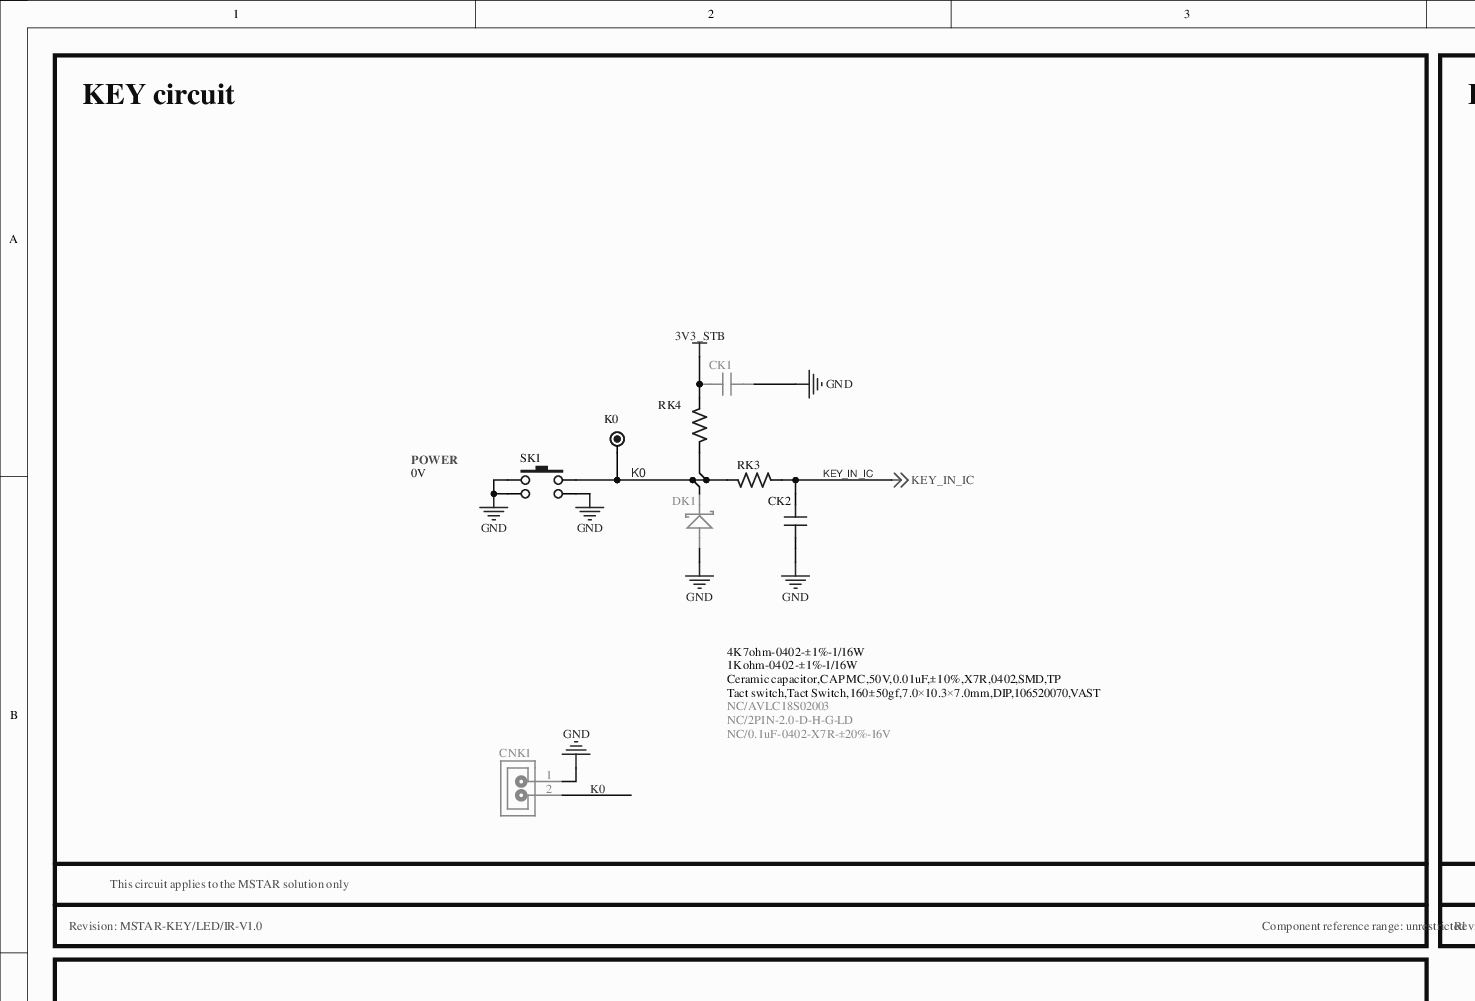
[diagram p0: MISC116569-8.SchDoc, top left]
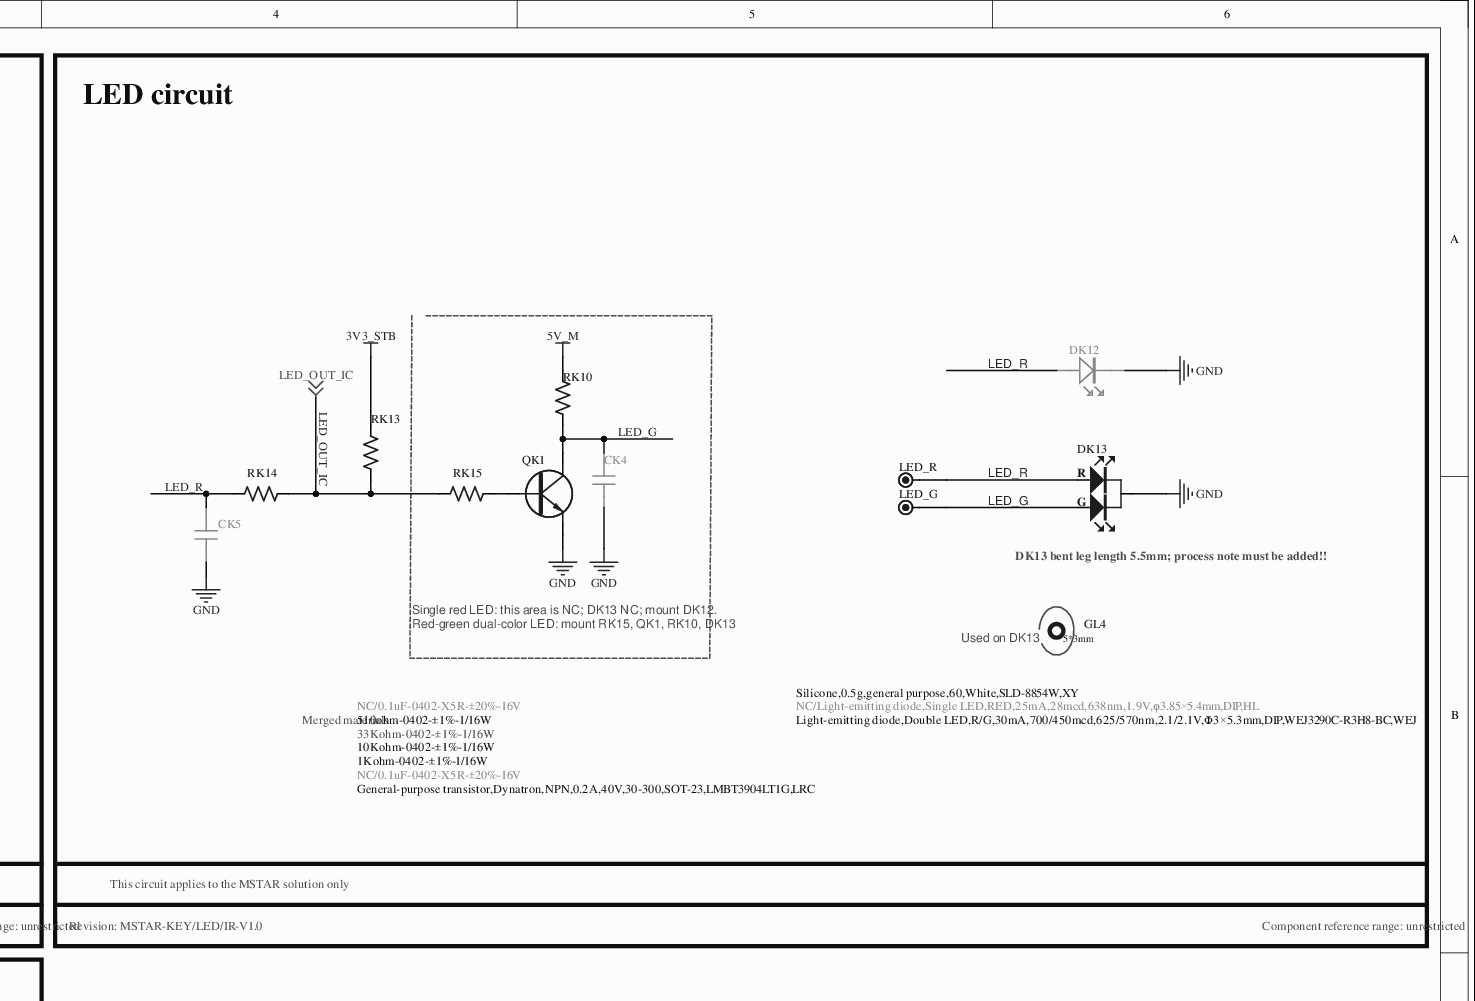
[diagram p1: MISC116569-8.SchDoc, top right]
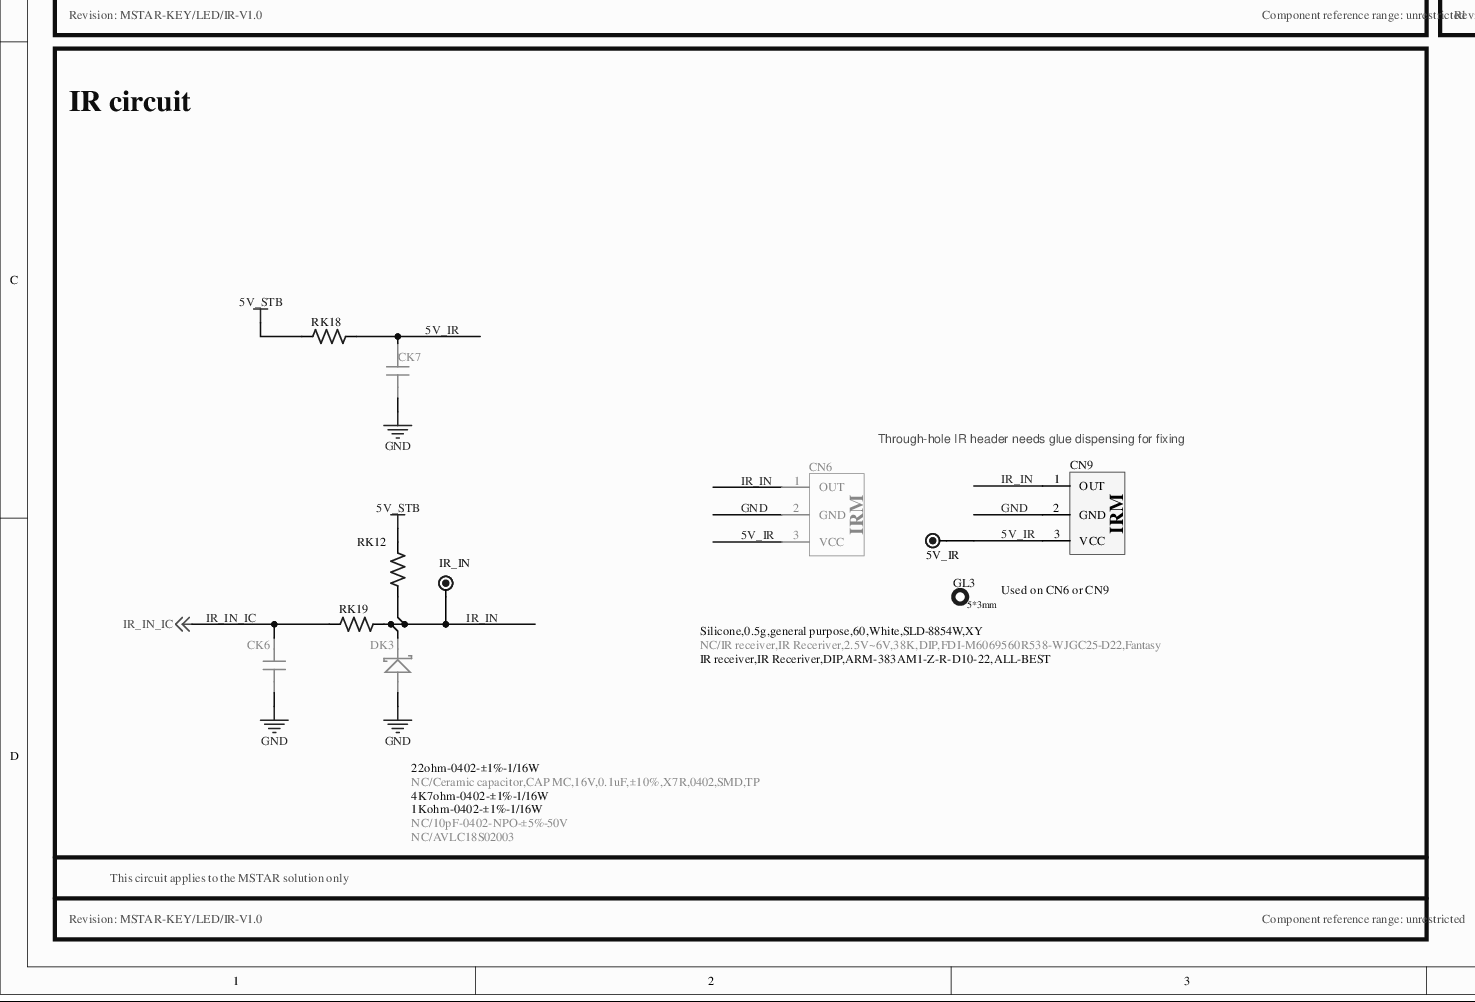
[diagram p2: MISC116569-8.SchDoc, bottom left]
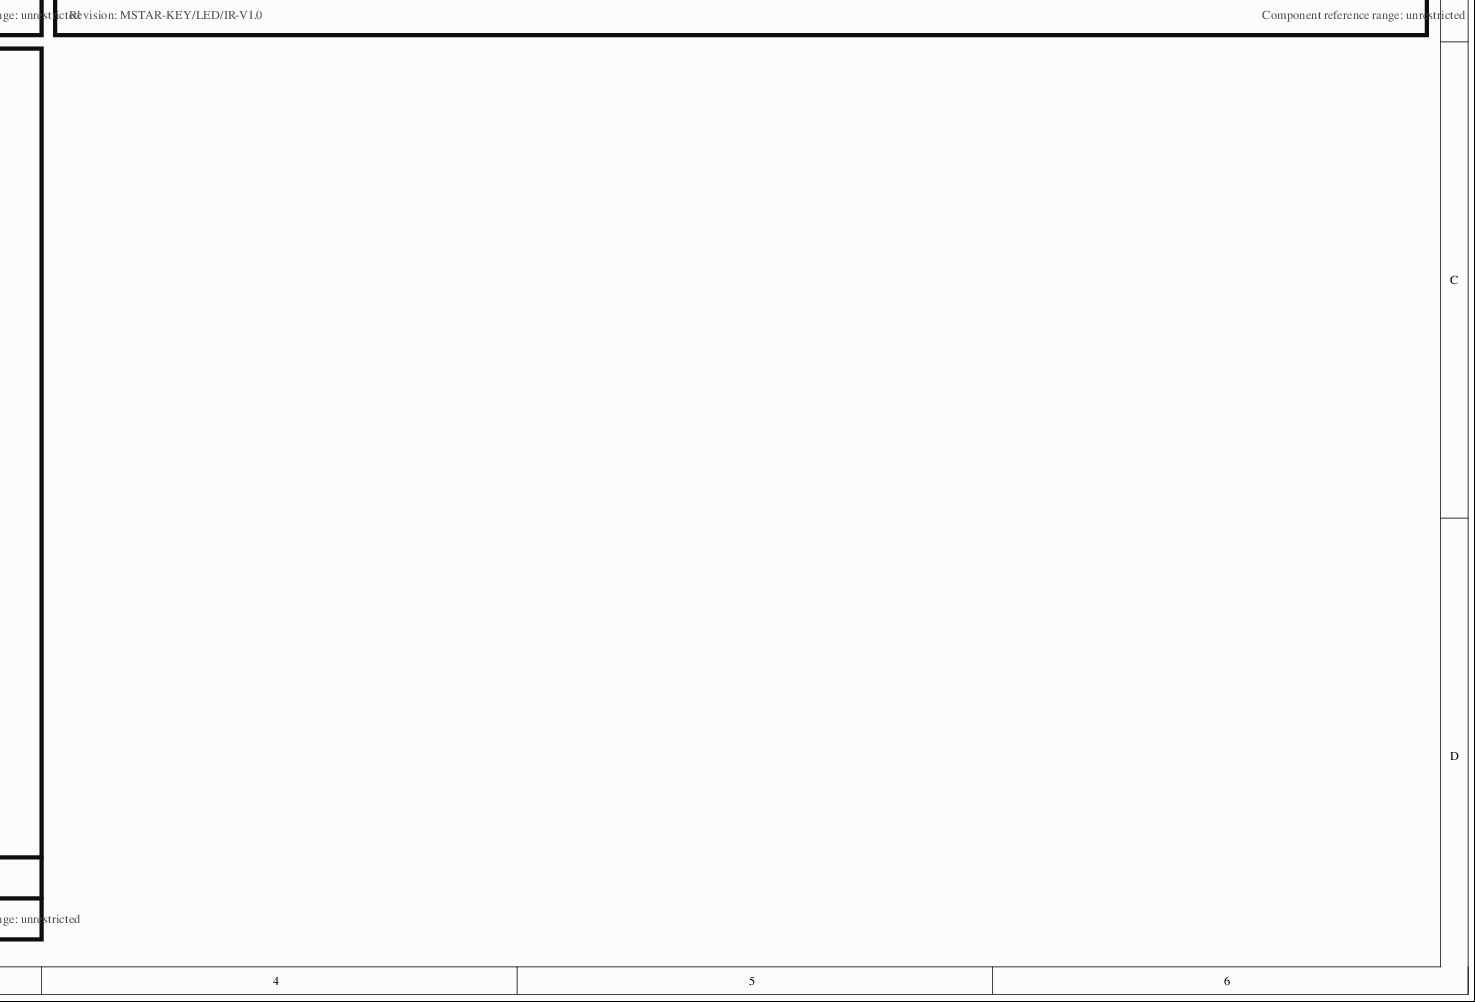
[diagram p3: MISC116569-8.SchDoc, bottom right]
# Altium project MISC116569-15.PrjPCB (part 4 of 8)

## Sheet MISC116569-8.SchDoc
size 528 x 353 mm

### Parts
5V_IR  TEST  SL  [TP]  (value not drawn)
CK1  NC/0.1uF-0402-X7R-±20%-16V  [C0402]
CK2  Ceramic capacitor,CAP MC,50V,0.01uF,±10%,X7R,0402,SMD,TP  [C0402]
CK4  NC/0.1uF-0402-X5R-±20%-16V  [C0402]
CK5  NC/0.1uF-0402-X5R-±20%-16V  [C0402]
CK6  NC/10pF-0402-NPO-±5%-50V  [C0402]
CK7  NC/Ceramic capacitor,CAP MC,16V,0.1uF,±10%,X7R,0402,SMD,TP  [C0402]
CN6  NC/IR receiver,IR Receriver,2.5V~6V,38K,DIP,FDI-M6069560R538-WJGC25-D22,Fantasy  [REMOTE-VD-9]
CN9  IR receiver,IR Receriver,DIP,ARM-383AM1-Z-R-D10-22,ALL-BEST  [REMOTE-VD-6]
CNK1  NC/2PIN-2.0-D-H-G-LD  [SIP2/2.0D-1]
DK1  NC/AVLC18S02003  [DIODE-S0402]
DK3  NC/AVLC18S02003  [DIODE-S0402]
DK12  NC/Light-emitting diode,Single LED,RED,25mA,28mcd,638nm,1.9V,φ3.85×5.4mm,DIP,HL  [LED-HD-6]
DK13  Light-emitting diode,Double LED,R/G,30mA,700/450mcd,625/570nm,2.1/2.1V,Φ3×5.3mm,DIP,WEJ3290C-R3H8-BC,WEJ  [LED-HD-5]
GL3  Silicone,0.5g,general purpose,60,White,SLD-8854W,XY  [Silica gel-5*3]
GL4  Silicone,0.5g,general purpose,60,White,SLD-8854W,XY  [Silica gel-5*3]
IR_IN  TEST  SL  [TP]  (value not drawn)
K0  TEST  SL  [TP]  (value not drawn)
LED_G  TEST  SL  [TP]  (value not drawn)
LED_R  TEST  SL  [TP]  (value not drawn)
QK1  General-purpose transistor,Dynatron,NPN,0.2A,40V,30-300,SOT-23,LMBT3904LT1G,LRC  [SOT-23]
RK3  1Kohm-0402-±1%-1/16W  [R0402]
RK4  4K7ohm-0402-±1%-1/16W  [R0402]
RK10  1Kohm-0402-±1%-1/16W  [R0402]
RK12  4K7ohm-0402-±1%-1/16W  [R0402]
RK13  33Kohm-0402-±1%-1/16W  [R0402]
RK14  510ohm-0402-±1%-1/16W  [R0402]
RK15  10Kohm-0402-±1%-1/16W  [R0402]
RK18  22ohm-0402-±1%-1/16W  [R0402]
RK19  1Kohm-0402-±1%-1/16W  [R0402]
SK1  Tact switch,Tact Switch,160±50gf,7.0×10.3×7.0mm,DIP,106520070,VAST  [KEY-HD-6]

### Blocks framed on the sheet
KEY circuit: CK1 CK2 CNK1 DK1 K0 RK3 RK4 SK1
LED circuit: CK4 CK5 DK12 DK13 GL4 LED_G LED_R QK1 RK10 RK13-RK15
IR circuit: 5V_IR CK6 CK7 CN6 CN9 DK3 GL3 IR_IN RK12 RK18 RK19

### Nets
3V3_STB: CK1.2 RK4.2 RK13.2
5V_M: RK10.2
5V_STB: RK12.2 RK18.2
GND: CK1.1 CK2.2 CK4.2 CK5.2 CK6.1 CK7.2 CN6.2(GND) CN9.2(GND) CNK1.1 DK1.A DK3.A DK12.K DK13.2 QK1.E SK1.1 SK1.3 SK1.4
5V_IR: 5V_IR.1 CK7.1 CN6.3(VCC) CN9.3(VCC) RK18.1
IR_IN: CN6.1(OUT) CN9.1(OUT) DK3.K IR_IN.1 RK12.1 RK19.1
IR_IN_IC: CK6.2 RK19.2 ; off-sheet IR_IN_IC
K0: CNK1.2 DK1.K K0.1 RK3.2 RK4.1 SK1.2
KEY_IN_IC: CK2.1 RK3.1 ; off-sheet KEY_IN_IC
LED_G: CK4.1 DK13.1 LED_G.1 QK1.C RK10.1
LED_OUT_IC: RK13.1 RK14.1 RK15.2 ; off-sheet LED_OUT_IC
LED_R: CK5.1 DK12.A DK13.3 LED_R.1 RK14.2
NetQK1_B: QK1.B RK15.1

### Notes on the sheet
- POWER
- 0V
- (near DK13) DK13 bent leg length 5.5mm; process note must be added!!
- Single red LED: this area is NC; DK13 NC; mount DK12.
- Red-green dual-color LED: mount RK15, QK1, RK10, DK13
- (near GL4) Used on DK13
- Merged materials
- This circuit applies to the MSTAR solution only
- Revision: MSTAR-KEY/LED/IR-V1.0
- Component reference range: unrestricted
- (near CN9) Through-hole IR header needs glue dispensing for fixing
- Used on CN6 or CN9

### Library data of the parts
CK1 = 0.1uF-0402-Y5V-+80%-20%-16V-D
CK2 = 0.01uF-0402-X7R-±10%-50V-D
CK4 CK5 = 0.1uF-0402-X5R-±20%-16V-D
CK6 = 10pF-0402-NPO-±5%-50V-D
CK7 = 1uF-0402-X5R-±20%-6.3V-D
CN6 = 004.008.0000361-DHMI: IR receiver,IR Receriver,2.5V~6V,38K,DIP,FDI-M6069560R538-WJGC25-D22,Fantasy-DHMI
CN9 = 004.008.0000501-DHMI: IR receiver,IR Receriver,DIP,ARM-383AW1-Z-R-D10-22,ALL-BEST-DHMI
CNK1 = 2PIN-2.0-D-H-G-B-DHMI: Socket
DK1 DK3 = AVLC18S02003-D
DK12 = 发光二极管,Single LED,RED,25mA,28mcd,638nm,1.9V,φ3.85×5.4mm,DIP,HL-DLMI
DK13 = WEJ3290C-R3H8-BC(红、绿)-高亮-DLMI
GL3 GL4 = 005.002.0000011-D-5*3mm: Silicone,0.5g,general purpose,60,White,SLD-8854W,XY-D
QK1 = LMBT3904LT1G-D-NPN: Q-NPN-#-#-#
RK3 RK10 = 1Kohm-0402-±5%-1/16W-D
RK4 = 4K7ohm-0402-±1%-1/16W-D
RK12 = 4K7ohm-0402-±5%-1/16W-D
RK13 = 33Kohm-0402-±5%-1/16W-D
RK14 = 510ohm-0402-±5%-1/16W-D
RK15 = 10Kohm-0402-±5%-1/16W-D
RK18 RK19 = 100ohm-0402-±5%-1/16W-D
SK1 = 轻触开关,Tact Switch,160±50gf,7.0×10.3×7.0mm,DIP,KFC-A06-E-4-7.5/4(R),YK-DLMI

## Sheet MISC116569-9.SchDoc
size 215 x 228 mm
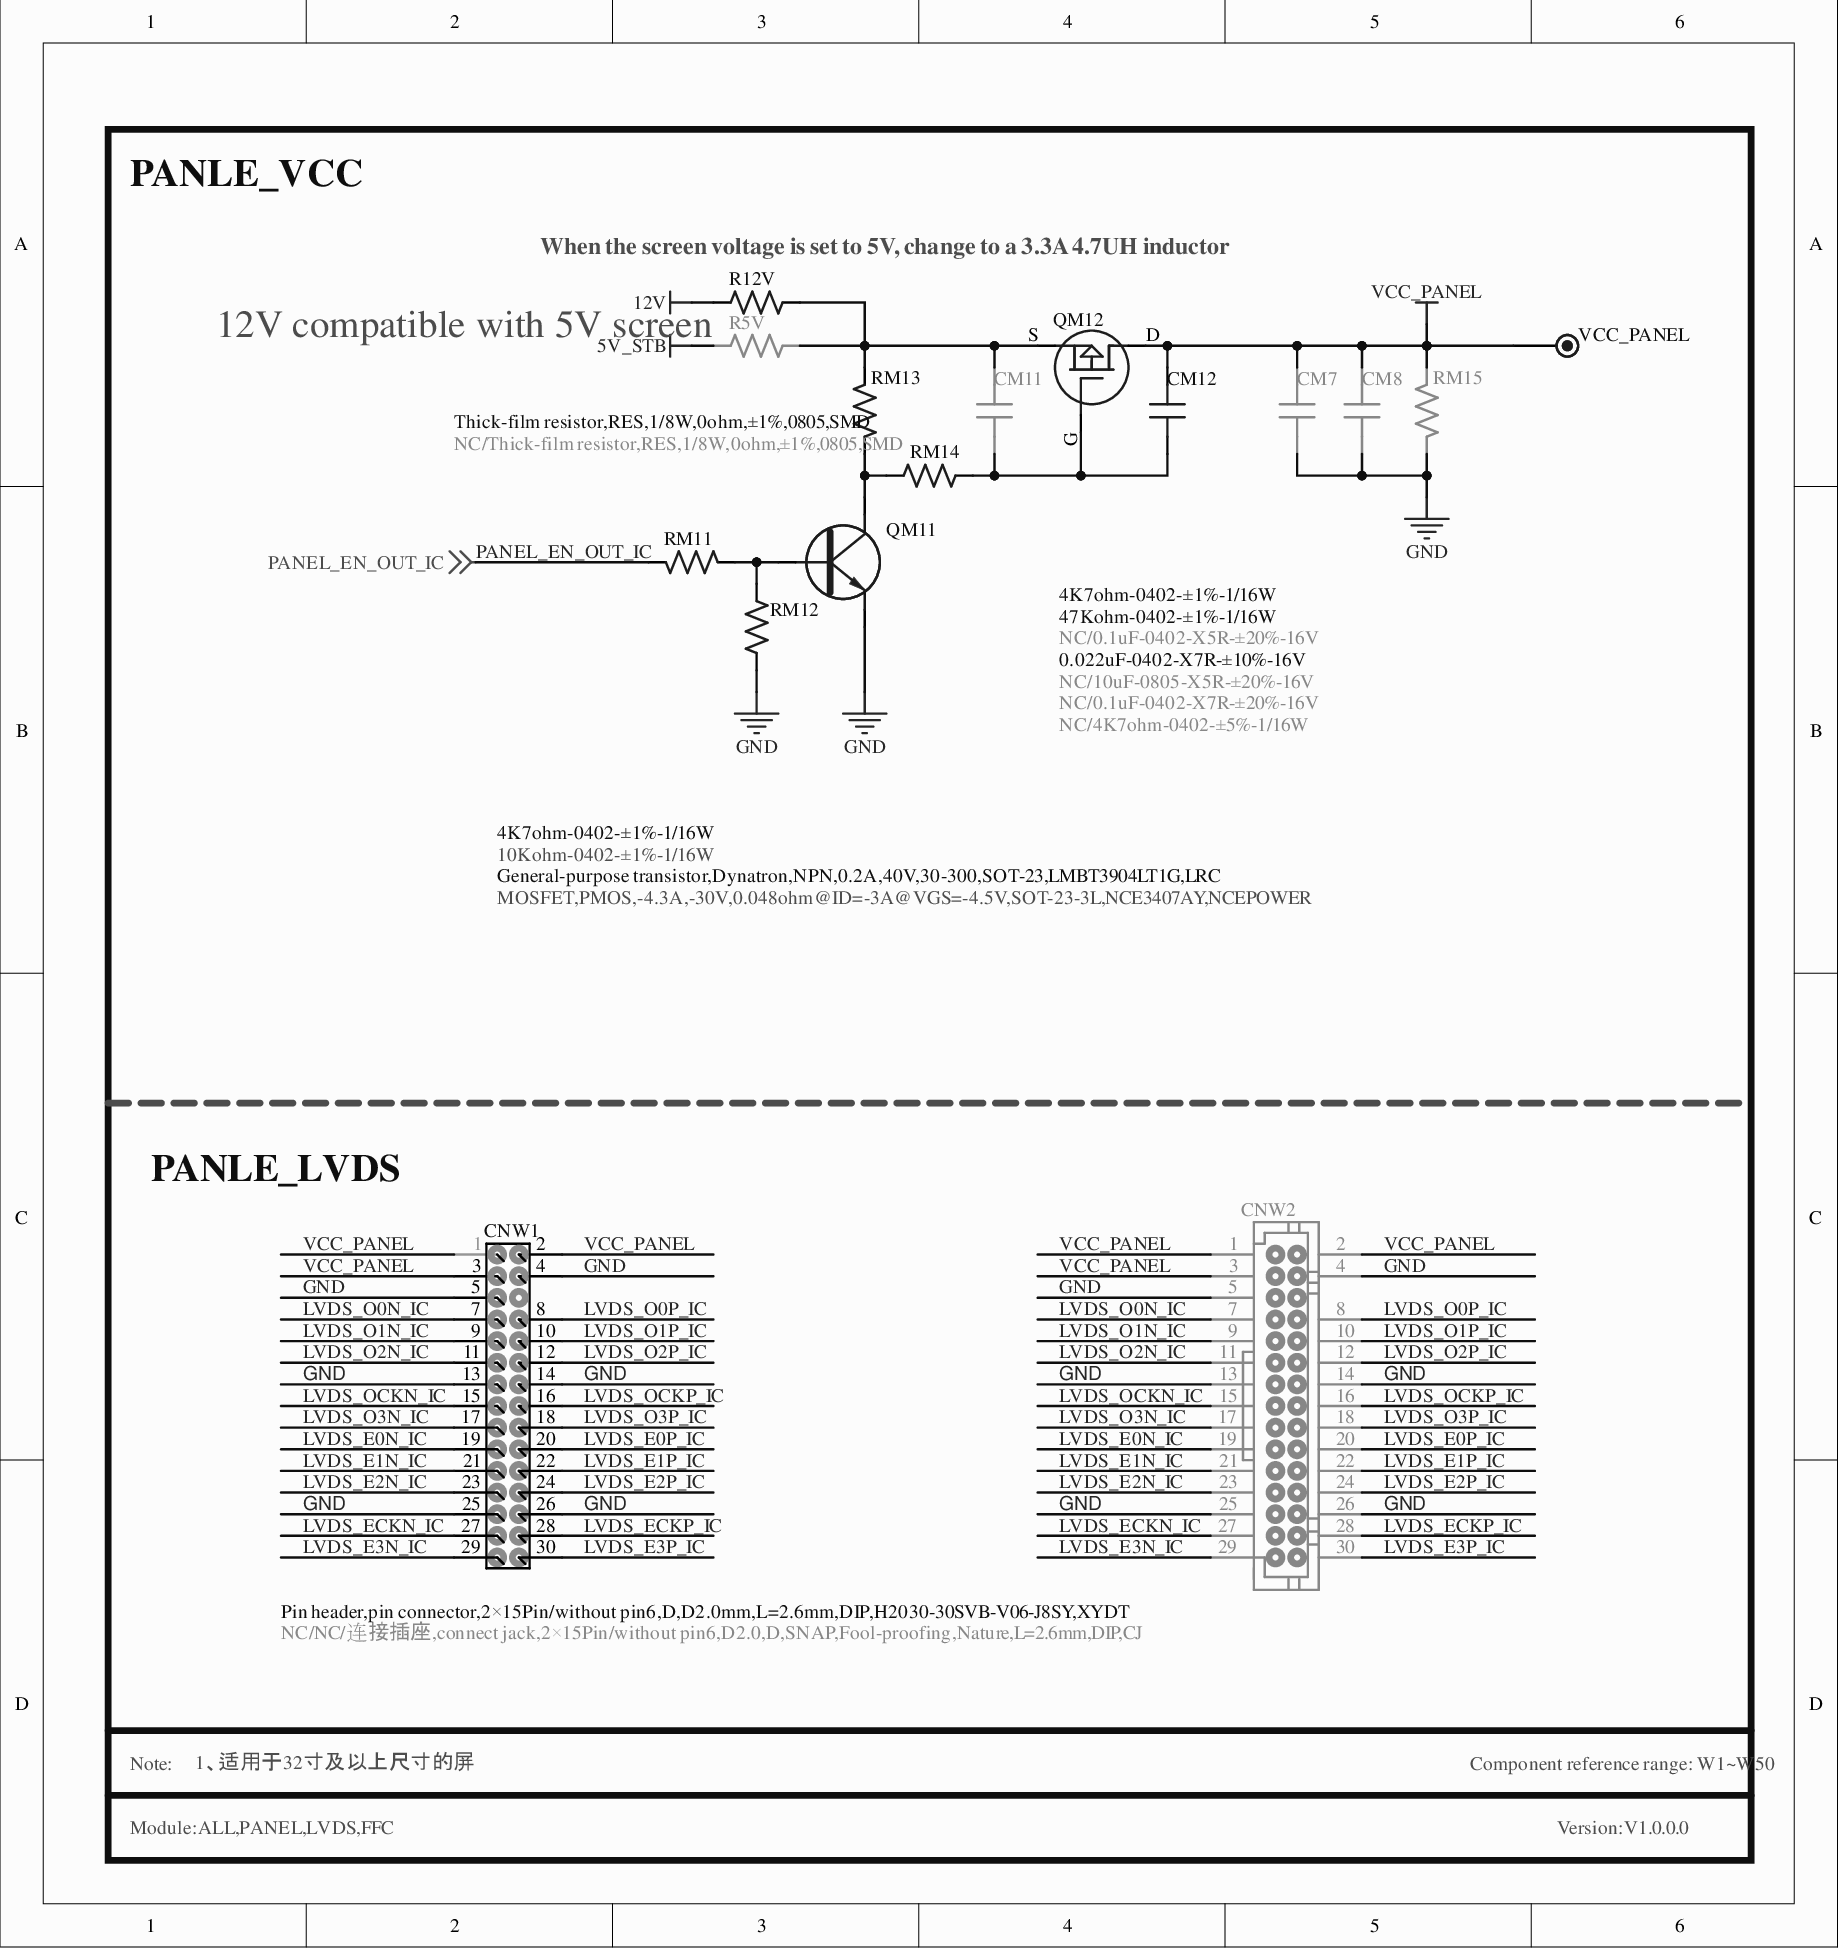
[diagram p4: MISC116569-9.SchDoc]

### Parts
CM7  NC/10uF-0805-X5R-±20%-16V  [C0805]
CM8  NC/0.1uF-0402-X7R-±20%-16V  [C0402]
CM11  NC/0.1uF-0402-X5R-±20%-16V  [C0402]
CM12  0.022uF-0402-X7R-±10%-16V  [C0402]
CNW1  Pin header,pin connector,2×15Pin/without pin6,D,D2.0mm,L=2.6mm,DIP,H2030-30SVB-V06-J8SY,XYDT  [SIP2*15/2.0D-2]
CNW2  NC/NC/连接插座,connect jack,2×15Pin/without pin6,D2.0,D,SNAP,Fool-proofing,Nature,L=2.6mm,DIP,CJ  [SIP2*15/2.0D-11]
QM11  General-purpose transistor,Dynatron,NPN,0.2A,40V,30-300,SOT-23,LMBT3904LT1G,LRC  [SOT-23]
QM12  MOSFET,PMOS,-4.3A,-30V,0.048ohm@ID=-3A@VGS=-4.5V,SOT-23-3L,NCE3407AY,NCEPOWER  [SOT-23-1]
R5V  NC/Thick-film resistor,RES,1/8W,0ohm,±1%,0805,SMD  [R0805]
R12V  Thick-film resistor,RES,1/8W,0ohm,±1%,0805,SMD  [R0805]
RM11  4K7ohm-0402-±1%-1/16W  [R0402]
RM12  10Kohm-0402-±1%-1/16W  [R0402]
RM13  4K7ohm-0402-±1%-1/16W  [R0402]
RM14  47Kohm-0402-±1%-1/16W  [R0402]
RM15  NC/4K7ohm-0402-±5%-1/16W  [R0402]
VCC_PANEL  TEST  [TP]  (value not drawn)

### Nets
5V_STB: R5V.1
12V: R12V.1
GND: CM7.2 CM8.1 CNW1.4 CNW1.5 CNW1.13 CNW1.14 CNW1.25 CNW1.26 CNW2.4 CNW2.5 CNW2.13 CNW2.14 CNW2.25 CNW2.26 QM11.E RM12.2 RM15.2
VCC_PANEL: CM7.1 CM8.2 CM12.1 CNW1.1 CNW1.2 CNW1.3 CNW2.1 CNW2.2 CNW2.3 QM12.D RM15.1 VCC_PANEL.1
LVDS_E0N_IC: CNW1.19 CNW2.19
LVDS_E0P_IC: CNW1.20 CNW2.20
LVDS_E1N_IC: CNW1.21 CNW2.21
LVDS_E1P_IC: CNW1.22 CNW2.22
LVDS_E2N_IC: CNW1.23 CNW2.23
LVDS_E2P_IC: CNW1.24 CNW2.24
LVDS_E3N_IC: CNW1.29 CNW2.29
LVDS_E3P_IC: CNW1.30 CNW2.30
LVDS_ECKN_IC: CNW1.27 CNW2.27
LVDS_ECKP_IC: CNW1.28 CNW2.28
LVDS_O0N_IC: CNW1.7 CNW2.7
LVDS_O0P_IC: CNW1.8 CNW2.8
LVDS_O1N_IC: CNW1.9 CNW2.9
LVDS_O1P_IC: CNW1.10 CNW2.10
LVDS_O2N_IC: CNW1.11 CNW2.11
LVDS_O2P_IC: CNW1.12 CNW2.12
LVDS_O3N_IC: CNW1.17 CNW2.17
LVDS_O3P_IC: CNW1.18 CNW2.18
LVDS_OCKN_IC: CNW1.15 CNW2.15
LVDS_OCKP_IC: CNW1.16 CNW2.16
PANEL_EN_OUT_IC: RM11.1 ; off-sheet PANEL_EN_OUT_IC
NetCM11_1: CM11.1 CM12.2 QM12.G RM14.2
NetCM11_2: CM11.2 QM12.S R5V.2 R12V.2 RM13.1
NetQM11_B: QM11.B RM11.2 RM12.1
NetQM11_C: QM11.C RM13.2 RM14.1

### Notes on the sheet
- PANLE_VCC
- (near R12V) When the screen voltage is set to 5V, change to a 3.3A 4.7UH inductor
- 12V compatible with 5V screen
- PANLE_LVDS
- Note:
- 1、适用于32寸及以上尺寸的屏
- Component reference range: W1~W50
- Module:ALL,PANEL,LVDS,FFC
- Version:V1.0.0.0

### Library data of the parts
CM7 = 004.003.0000386-D: Ceramic capacitor,CAP MC,16V,10uF,±20%,X5R,0805,SMD,TP-D
CM8 = 004.003.0000403-D: Ceramic capacitor,CAP MC,16V,0.1uF,±20%,X5R,0402,SMD,TP-D
CM11 = 0.1uF-0402-X5R-±20%-16V-D
CM12 = 0.022uF-0402-X7R-±10%-16V-D
CNW1 = 2×15PIN-2.0-D-H-M(脚长=2.6mm)(缺6PIN)-LK-DHMI: CN-straight pin header
CNW2 = 连接插座,connect jack,2×15Pin/without pin6,D2.0,D,SNAP,Fool-proofing,Nature,L=2.6mm,DIP,CJ: CN-with latch
QM11 = LMBT3904LT1G-D-NPN: Q-NPN-#-#-#
QM12 = WPM3407C-3/TR-D
R5V R12V = 0ohm-0805-±5%-1/8W-D
RM11 RM13 RM15 = 4K7ohm-0402-±5%-1/16W-D
RM12 = 10Kohm-0402-±5%-1/16W-D
RM14 = 47Kohm-0402-±5%-1/16W-D